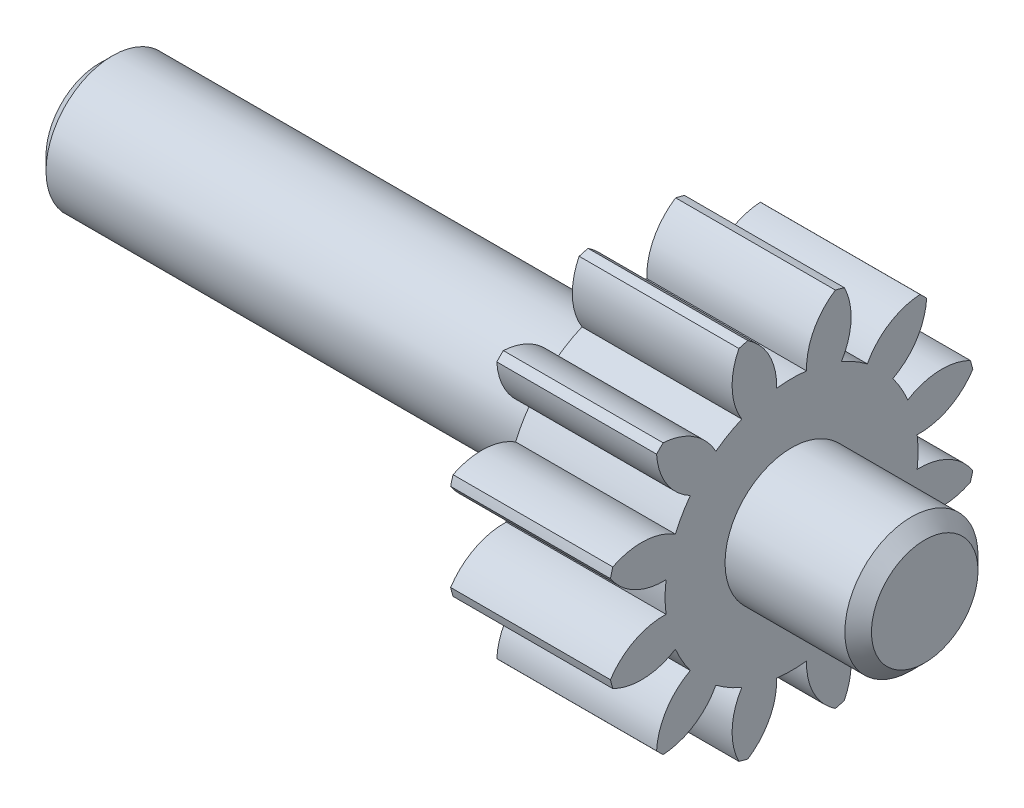
from build123d import *

# Parameters (mm, degrees)
BASPROSKE_W         = 6
BASPROSKE_H         = 7
TOOTHCUT_DEPTH      = 12.575836903
TEETHCUTS_COUNT     = 12
TEETHCUTS_ANGLE     = 330
BORSKE_R            = 0.4
BORE_DEPTH          = 50.0000508
SKETCH1_R           = 2.5
BOSS_EXTRUDE1_DEPTH = 5
BOSS_EXTRUDE2_START = 20
SKETCH2_R           = 2.5
BOSS_EXTRUDE2_DEPTH = 20
CHAMFER1_SIZE       = 0.5


with BuildPart() as part:
    # BasProSke → Base-Revolve (revolve)
    with BuildSketch(Plane(origin=(0, 0, 0), x_dir=(1, 0, 0), z_dir=(0, 1, 0)), mode=Mode.PRIVATE) as base_revolve_sk:
        with Locations((3, 3.5)):
            Rectangle(BASPROSKE_W, BASPROSKE_H)
    revolve(base_revolve_sk.sketch.rotate(Axis((-10, 0, 0), (1, 0, 0)), 180), axis=Axis((-10, 0, 0), (1, 0, 0)))

    # TooCutSke → ToothCut (cut, through all)
    with BuildSketch(Plane(origin=(0, 0, 0), x_dir=(0, 0, -1), z_dir=(1, 0, 0))):
        with BuildLine():
            ThreePointArc((0.562207301, 4.715604304), (0, 4.749), (-0.562207301, 4.715604304))
            ThreePointArc((-0.562207301, 4.715604304), (-0.837528627, 5.917009812), (-1.672850686, 6.823328788))
            ThreePointArc((-1.672850686, 6.823328788), (0, 7.0254), (1.672850686, 6.823328788))
            ThreePointArc((1.672850686, 6.823328788), (0.837528627, 5.917009812), (0.562207301, 4.715604304))
        make_face()
    toothcut = extrude(amount=TOOTHCUT_DEPTH, mode=Mode.SUBTRACT)

    # TeethCuts: ToothCut ×12 about axis
    teethcuts_axis = Axis((-10, 0, 0), (1, 0, 0))
    for i in range(1, TEETHCUTS_COUNT):
        add(toothcut.rotate(teethcuts_axis, i * TEETHCUTS_ANGLE / (TEETHCUTS_COUNT - 1)), mode=Mode.SUBTRACT)

    # BorSke → Bore (cut, symmetric)
    with BuildSketch(Plane(origin=(0, 0, 0), x_dir=(0, 0, -1), z_dir=(1, 0, 0))):
        with Locations(Location((0, 0, 0), (0, 0, 180))):
            Circle(BORSKE_R)
    extrude(amount=BORE_DEPTH, both=True, mode=Mode.SUBTRACT)

    # Sketch1 → Boss-Extrude1 (add)
    with BuildSketch(Plane(origin=(6, 0, 0), x_dir=(0, 0, -1), z_dir=(1, 0, 0))):
        with Locations(Location((0, 0, 0), (0, 0, 180))):
            Circle(SKETCH1_R)
    extrude(amount=BOSS_EXTRUDE1_DEPTH)

    # Sketch2 → Boss-Extrude2 (add)
    with BuildSketch(Plane.ZY.offset(BOSS_EXTRUDE2_START)):
        Circle(SKETCH2_R)
    extrude(amount=-BOSS_EXTRUDE2_DEPTH)

    # Chamfer1
    chamfer1_edges = [part.edges().sort_by_distance(p)[0] for p in [
        (11, 0, -2.5),
        (-20, 0, -2.5),
    ]]
    chamfer(chamfer1_edges, length=CHAMFER1_SIZE)


solid = part.part
